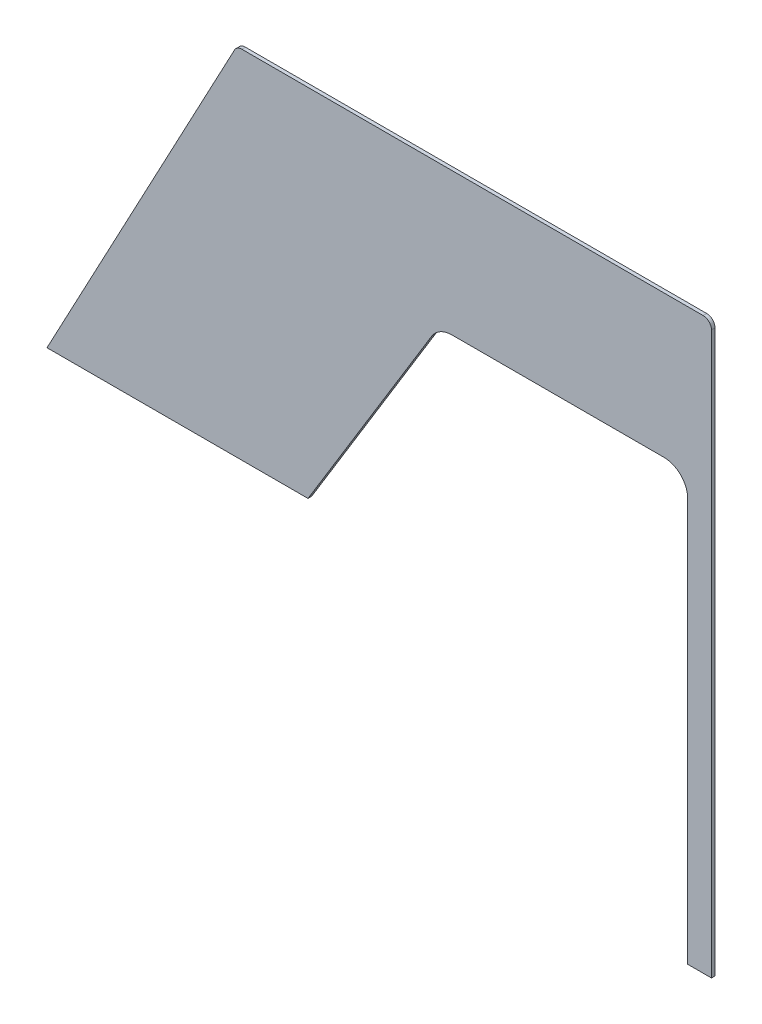
SolidWorks part; units mm, degrees
material "1023 Carbon Steel Plate (SS)"
ref_plane "Front Plane" through (0, 0, 0) normal (0, 0, 1) x (1, 0, 0)
ref_plane "Top Plane" through (0, 0, 0) normal (0, 1, 0) x (1, 0, 0)
ref_plane "Right Plane" through (0, 0, 0) normal (1, 0, 0) x (0, 0, -1)
sketch "Sketch1" plane through (0, 0, 0) normal (0, 0, 1) x (1, 0, 0)
  line L0 (0, 0) -> (79.0118, 148.1471)
  line L1 (82.1, 150) -> (276.5, 150)
  line L2 (280, 146.5) -> (280, -90)
  line L3 (280, -90) -> (270, -90)
  line L4 (270, -90) -> (270, 80)
  line L5 (260, 90) -> (170.6083, 90)
  line L6 (162.0755, 85.2145) -> (110, 0)
  line L7 (110, 0) -> (0, 0)
  arc A0 (276.5, 150) -> (280, 146.5) centre (276.5, 146.5) cw
  arc A1 (79.0118, 148.1471) -> (82.1, 150) centre (82.1, 146.5) cw
  arc A2 (270, 80) -> (260, 90) centre (260, 80) ccw
  arc A3 (170.6083, 90) -> (162.0755, 85.2145) centre (170.6083, 80) ccw
  point P12 (280, 150)
  point P15 (80, 150)
  point P18 (270, 90)
  point P21 (165, 90)
  dimension "D9" = 3.5
  dimension "D10" = 10
  dimension "D1" = 80
  dimension "D2" = 200
  dimension "D3" = 10
  dimension "D4" = 160
  dimension "D5" = 105
  dimension "D6" = 150
  dimension "D7" = 90
  dimension "D8" = 240
extrude "Boss-Extrude1" add sketch "Sketch1" along normal blind 1.5 contours L7 L0 A1 L1 A0 L2 L3 L4 A2 L5 A3 L6
